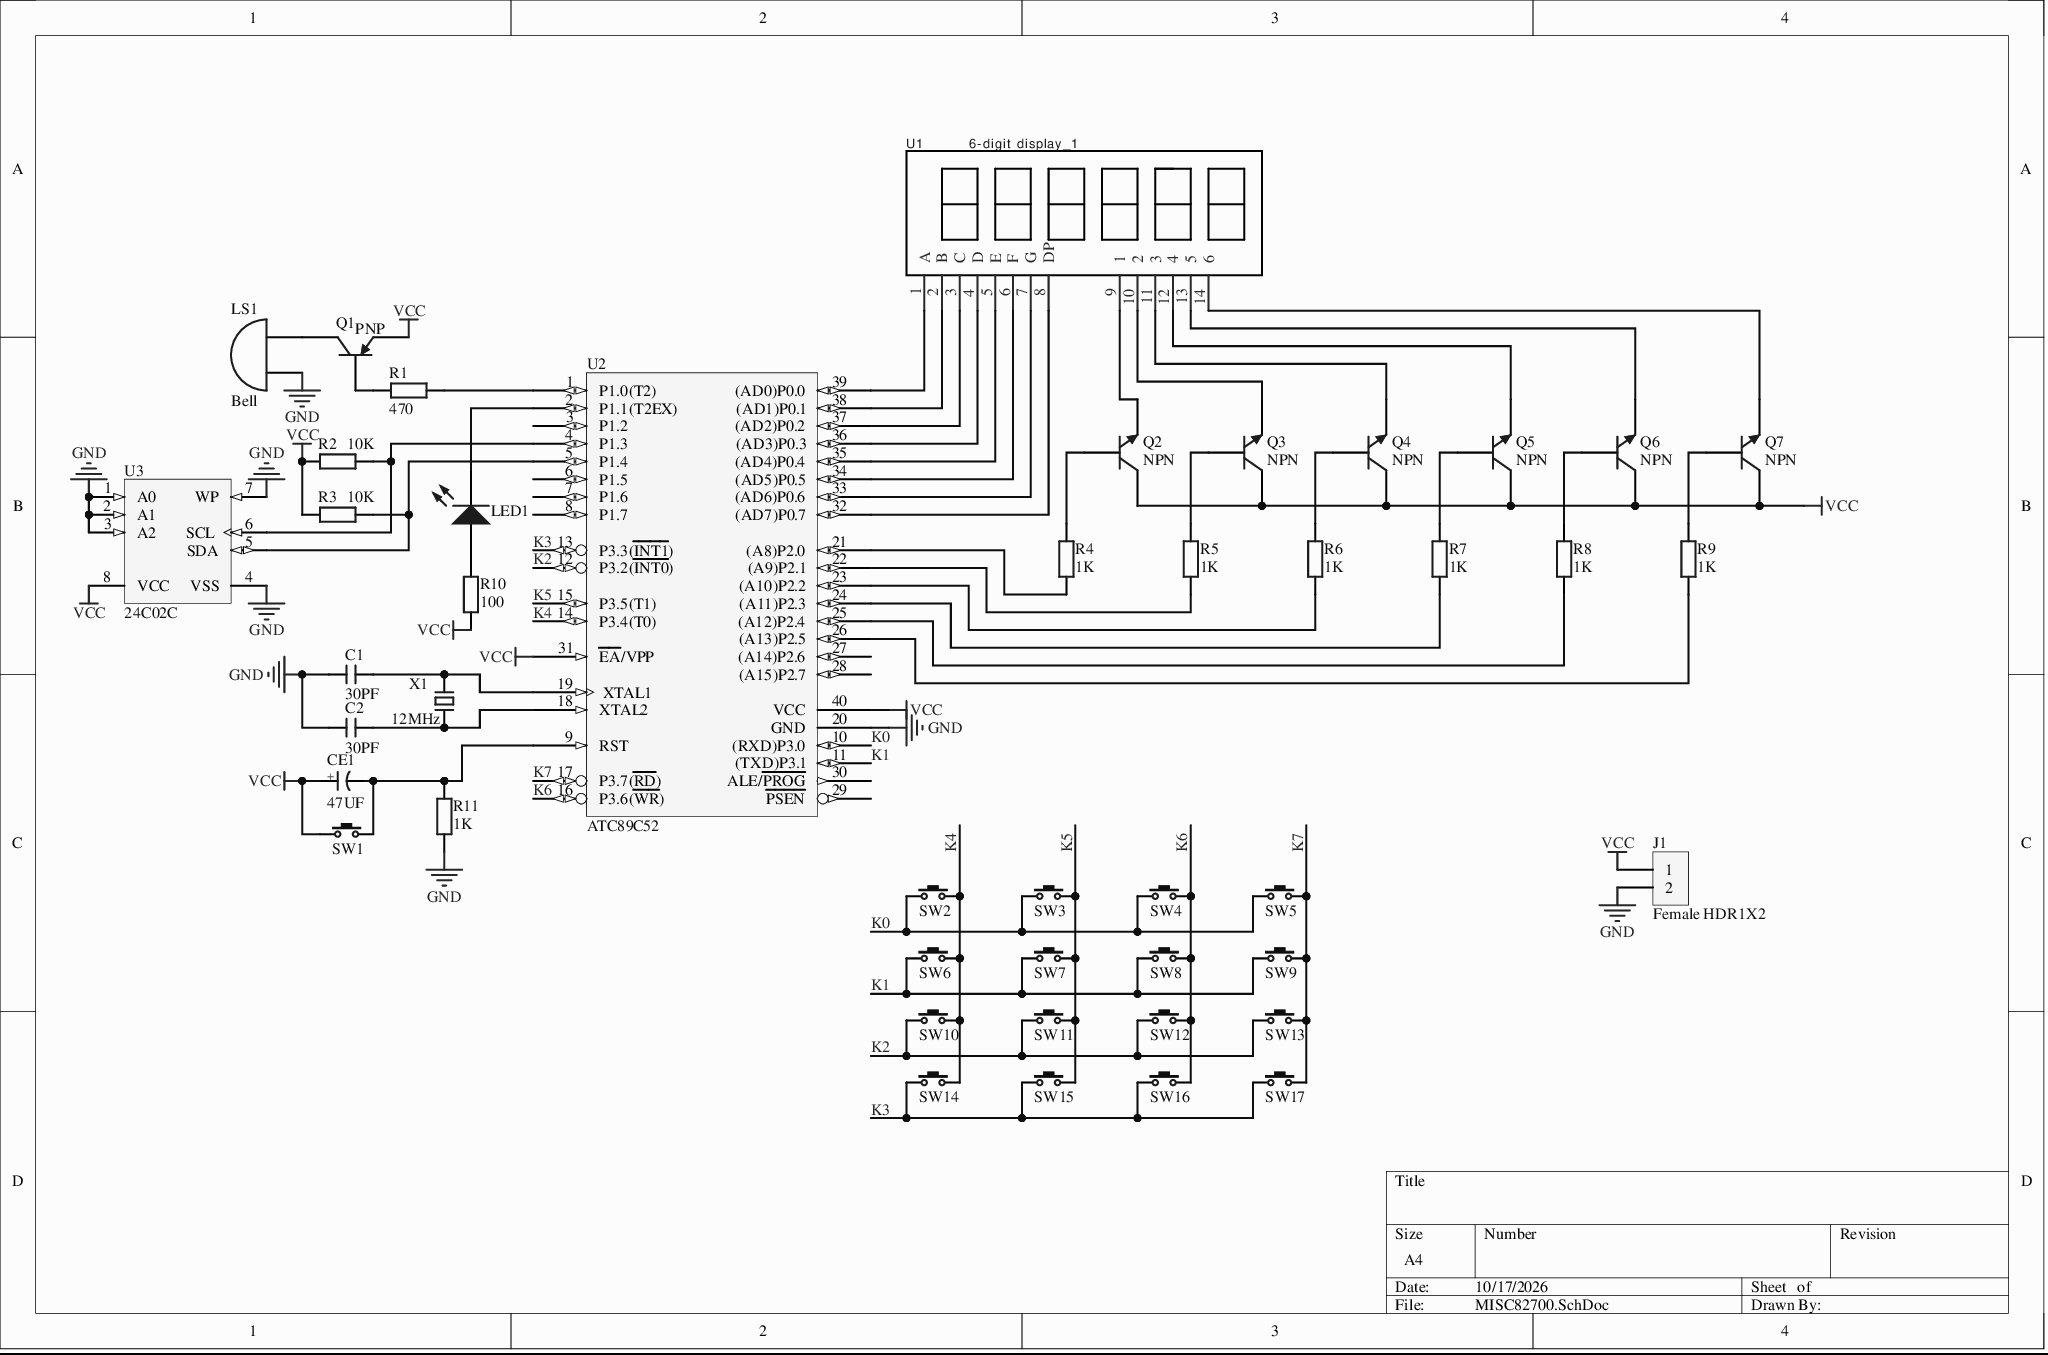
[diagram p0: MISC82700.SchDoc]
# Altium project MISC82700.PrjPcb
1 sheet, 45 parts. Net scope: global (net labels, ports and power ports of the same name join across sheets).
Board file: MISC82700.PcbDoc

## Sheet MISC82700.SchDoc
size A4

### Parts
C1  30PF  [CC 1.8*3.6]
C2  30PF  [CC 1.8*3.6]
CE1  47UF  [CAP 1.5*4*8]
J1  Female HDR1X2  [Fe-HDR1X2/2.54-S]
LED1  Red  [LED 5MM-B]  (value not drawn)
LS1  Bell  [PIN2]
Q1  PNP  [TO-92A]
Q2  NPN  [TO-226-AA]
Q3  NPN  [TO-226-AA]
Q4  NPN  [TO-226-AA]
Q5  NPN  [TO-226-AA]
Q6  NPN  [TO-226-AA]
Q7  NPN  [TO-226-AA]
R1  470  [RS 1/4W]
R2  10K  [RS 1/4W]
R3  10K  [RS 1/4W]
R4  1K  [RS 1/4W]
R5  1K  [RS 1/4W]
R6  1K  [RS 1/4W]
R7  1K  [RS 1/4W]
R8  1K  [RS 1/4W]
R9  1K  [RS 1/4W]
R10  100  [RS 1/4W]
R11  1K  [RS 1/4W]
SW1  3x6x5  [四脚轻触开关]  (value not drawn)
SW2  3x6x5  [四脚轻触开关]  (value not drawn)
SW3  3x6x5  [四脚轻触开关]  (value not drawn)
SW4  3x6x5  [四脚轻触开关]  (value not drawn)
SW5  3x6x5  [四脚轻触开关]  (value not drawn)
SW6  3x6x5  [四脚轻触开关]  (value not drawn)
SW7  3x6x5  [四脚轻触开关]  (value not drawn)
SW8  3x6x5  [四脚轻触开关]  (value not drawn)
SW9  3x6x5  [四脚轻触开关]  (value not drawn)
SW10  3x6x5  [四脚轻触开关]  (value not drawn)
SW11  3x6x5  [四脚轻触开关]  (value not drawn)
SW12  3x6x5  [四脚轻触开关]  (value not drawn)
SW13  3x6x5  [四脚轻触开关]  (value not drawn)
SW14  3x6x5  [四脚轻触开关]  (value not drawn)
SW15  3x6x5  [四脚轻触开关]  (value not drawn)
SW16  3x6x5  [四脚轻触开关]  (value not drawn)
SW17  3x6x5  [四脚轻触开关]  (value not drawn)
U1  6-digit display_1  [6位数码管]
U2  ATC89C52  [DIP40]
U3  24C02C  [PDIP300-P8]
X1  12MHz  [OSC HC-49S]

### Nets
GND: C1.1 C2.1 J1.2 LS1.1(A) R11.1 U2.20(GND) U3.1(A0) U3.2(A1) U3.3(A2) U3.4(VSS) U3.7(WP)
VCC: CE1.1(A) J1.1 Q1.1(E) Q2.1(C) Q3.1(C) Q4.1(C) Q5.1(C) Q6.1(C) Q7.1(C) R2.2 R3.2 R10.2 SW1.1 U2.31(~{EA}/VPP) U2.40(VCC) U3.8(VCC)
K0: SW2.1 SW3.1 SW4.1 SW5.1 U2.10((RXD)P3.0)
K1: SW6.1 SW7.1 SW8.1 SW9.1 U2.11((TXD)P3.1)
K2: SW10.1 SW11.1 SW12.1 SW13.1 U2.12(P3.2(~{INT0}))
K3: SW14.1 SW15.1 SW16.1 SW17.1 U2.13(P3.3(~{INT1}))
K4: SW2.2 SW6.2 SW10.2 SW14.2 U2.14(P3.4(T0))
K5: SW3.2 SW7.2 SW11.2 SW15.2 U2.15(P3.5(T1))
K6: SW4.2 SW8.2 SW12.2 SW16.2 U2.16(P3.6(~{WR}))
K7: SW5.2 SW9.2 SW13.2 SW17.2 U2.17(P3.7(~{RD}))
NetC1_2: C1.2 U2.19(XTAL1) X1.2
NetC2_2: C2.2 U2.18(XTAL2) X1.1
NetCE1_2: CE1.2(K) R11.2 SW1.2 U2.9(RST)
NetLED1_1: LED1.1(A) R10.1
NetLED1_2: LED1.2(K) U2.2(P1.1(T2EX))
NetLS1_2: LS1.2(B) Q1.3(C)
NetQ1_2: Q1.2(B) R1.2
NetQ2_2: Q2.2(B) R4.2
NetQ2_3: Q2.3(E) U1.9(1)
NetQ3_2: Q3.2(B) R5.2
NetQ3_3: Q3.3(E) U1.10(2)
NetQ4_2: Q4.2(B) R6.2
NetQ4_3: Q4.3(E) U1.11(3)
NetQ5_2: Q5.2(B) R7.2
NetQ5_3: Q5.3(E) U1.12(4)
NetQ6_2: Q6.2(B) R8.2
NetQ6_3: Q6.3(E) U1.13(5)
NetQ7_2: Q7.2(B) R9.2
NetQ7_3: Q7.3(E) U1.14(6)
NetR1_1: R1.1 U2.1(P1.0(T2))
NetR2_1: R2.1 U2.4(P1.3) U3.6(SCL)
NetR3_1: R3.1 U2.5(P1.4) U3.5(SDA)
NetR4_1: R4.1 U2.21((A8)P2.0)
NetR5_1: R5.1 U2.22((A9)P2.1)
NetR6_1: R6.1 U2.23((A10)P2.2)
NetR7_1: R7.1 U2.24((A11)P2.3)
NetR8_1: R8.1 U2.25((A12)P2.4)
NetR9_1: R9.1 U2.26((A13)P2.5)
NetU1_1: U1.1(A) U2.39((AD0)P0.0)
NetU1_2: U1.2(B) U2.38((AD1)P0.1)
NetU1_3: U1.3(C) U2.37((AD2)P0.2)
NetU1_4: U1.4(D) U2.36((AD3)P0.3)
NetU1_5: U1.5(E) U2.35((AD4)P0.4)
NetU1_6: U1.6(F) U2.34((AD5)P0.5)
NetU1_7: U1.7(G) U2.33((AD6)P0.6)
NetU1_8: U1.8(DP) U2.32((AD7)P0.7)

Not connected (* = marked no-connect by the designer): U2 3(P1.2) 6(P1.5) 7(P1.6) 8(P1.7) 27((A14)P2.6) 28((A15)P2.7) 29(~{PSEN}) 30(ALE/~{PROG})

### Library data of the parts
C1 C2 = CC: Ceramic capacitor; BOM名称: Through-hole ceramic capacitor
CE1 = CE: Through-hole electrolytic capacitor; BOM名称: Through-hole electrolytic capacitor
LED1 = LED-5MM: 5mm through-hole LED; BOM名称: 5mm through-hole LED
LS1 = Bell: Electrical Bell; Published: 24-Mar-1999; LatestRevisionDate: 17-Jul-2002; LatestRevisionNote: Re-released for DXP Platform.; PackageReference: PIN2; Publisher: Altium Limited
Q1 = 2N3906: PNP General Purpose Amplifier; Published: 8-Jun-2000; LatestRevisionDate: 15-Jan-2003; LatestRevisionNote: PCB Footprint 'BCY-W3/D4.7' replaced; DatasheetVersion: 1997; PackageVersion: Sep-1998; PackageReference: TO-92A; PackageDescription: TO, Flat Index; 3 In-Line, Axial Leads; Body Dia. 4.5mm; Leads 0.51 x 0.48 mm (max); ComponentLink1Description: Manufacturer Link; ComponentLink2Description: Datasheet; ComponentLink2URL: http://www.fairchildsemi.com/ds/2N%2F2N3906.pdf; Publisher: Altium Limited
Q2-Q7 = NPN: NPN Bipolar Transistor; Published: 8-Jun-2000; LatestRevisionDate: 17-Jul-2002; LatestRevisionNote: Re-released for DXP Platform.; PackageReference: TO-226-AA; PackageDescription: TO, Flat Index; 3 In-Line, Axial Leads; Body Dia. 4.8mm; Leads 0.55 x 0.51 mm (max); Code_JEDEC: TO-226-AA; Publisher: Altium Limited
R1-R11 = R-S: Color-band resistor; BOM名称: Color-band resistor
SW1-SW17 = TSW 3x6: 3x6 tactile switch; BOM名称: 3x6 tactile switch
U1 = 6位数码管_1
U2 = STC89C52
U3 = 24C02C-I/P: 2Kbit, 400kHz, 5V, I2C Serial EEPROM, 8-Pin PDIP, Industrial Temperature; Published: 29-Jan-2009; DatasheetVersion: revJ, Aug-2008; PackageVersion: revBB, Aug-2009; PackageReference: PDIP300-P8; PackageDescription: 8-Lead Plastic Dual In-Line (P) - 300 mil Body [PDIP]; Supplier 1: Digi-Key; Supplier Part Number 1: 24C02C-I/P-ND; Supplier 2: Farnell; Supplier Part Number 2: 1755843; Code_JEDEC: MS-001; ComponentLink1Description: Datasheet; ComponentLink1URL: http://ww1.microchip.com/downloads/en/DeviceDoc/21202J.pdf; ComponentLink2Description: Packaging Specification; ComponentLink2URL: http://www.microchip.com/stellent/groups/techpub_sg/documents/packagingspec/en012702.pdf; ComponentLink3Description: Microchip.com Home; Publisher: Altium Limited
X1 = XTAL-2P: 2-pin passive crystal; BOM名称: 2-pin passive crystal